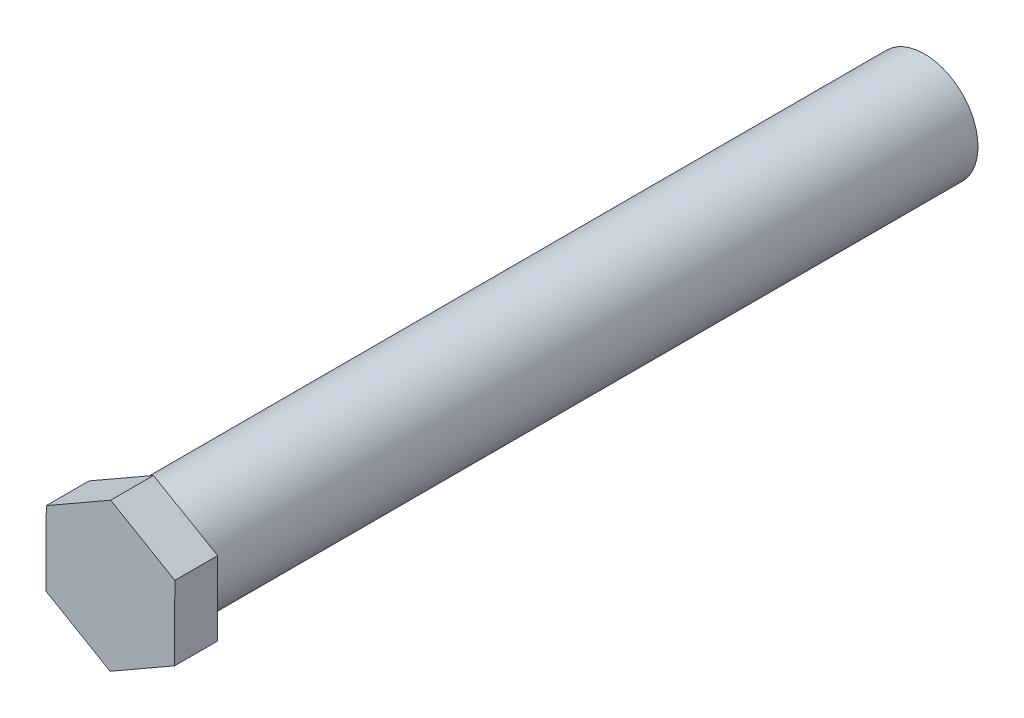
SolidWorks part; units mm, degrees
ref_plane "前视基准面" through (0, 0, 0) normal (0, 0, 1) x (1, 0, 0)
ref_plane "上视基准面" through (0, 0, 0) normal (0, 1, 0) x (1, 0, 0)
ref_plane "右视基准面" through (0, 0, 0) normal (1, 0, 0) x (0, 0, -1)
sketch "草图1" plane through (0, 0, 0) normal (0, 0, 1) x (1, 0, 0)
  circle A0 centre (0, 0) radius 5
  dimension "D1" = 10
extrude "凸台-拉伸1" add sketch "草图1" along normal blind 72
cosmetic thread "装饰螺纹线1" parameters "D2"=9
sketch "草图2" plane through (0, 0, 72) normal (0, 0, 1) x (1, 0, 0)
  line L1 (5.9872, -3.4861) -> (6.0127, 3.442)
  line L2 (6.0127, 3.442) -> (0.0255, 6.9282)
  line L3 (0.0255, 6.9282) -> (-5.9872, 3.4861)
  line L4 (-5.9872, 3.4861) -> (-6.0127, -3.442)
  line L5 (-6.0127, -3.442) -> (-0.0255, -6.9282)
  line L6 (-0.0255, -6.9282) -> (5.9872, -3.4861)
  circle A0 centre (0, 0) radius 6 construction
  dimension "D1" = 12
extrude "凸台-拉伸2" add sketch "草图2" along normal blind 4
